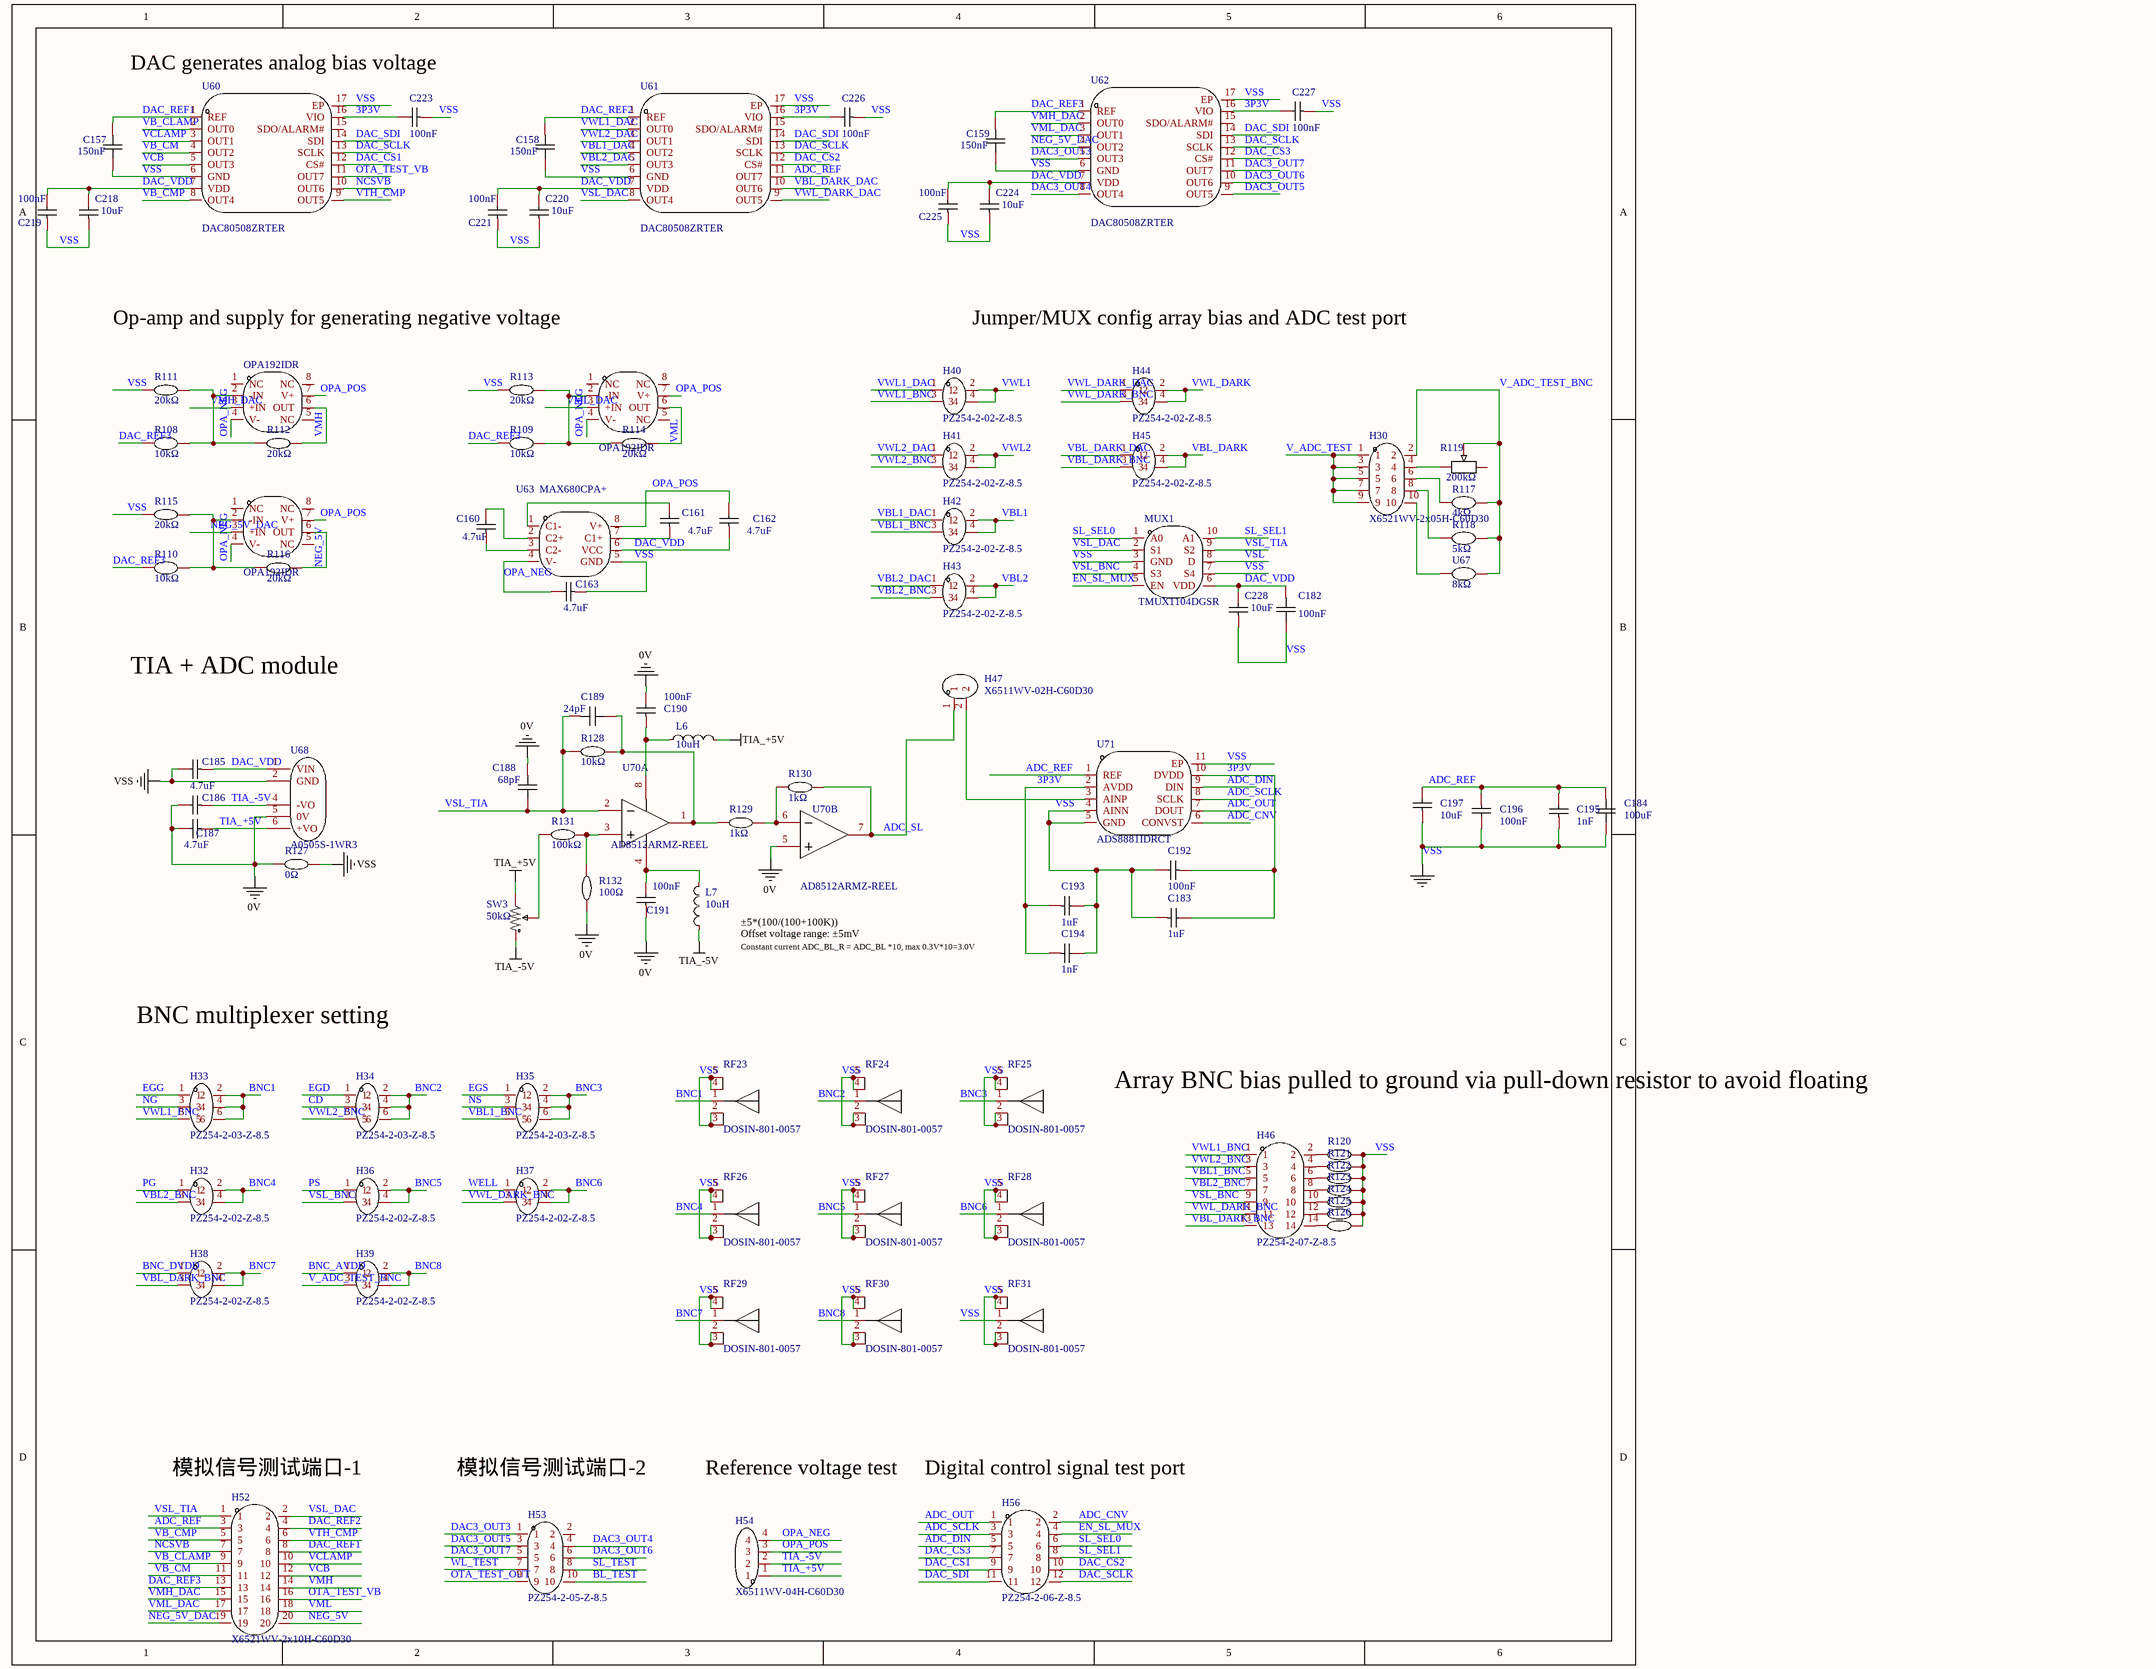
[diagram p0: MISC62793-4.schdoc]
# Altium project MISC62793-14.PrjPcb (part 3 of 4)
## Sheet MISC62793-4.schdoc (continued)
### Library data of the parts (continued)
R108-R110 = RT0603BRD0710KL: Manufacturer: YAGEO(国巨); Symbol: 1.25kΩ; Add into BOM: yes; Tolerance: ±0.1%; Power(Watts): 100mW; Overload Voltage (Max): 75V; Temperature Coefficient: ±25ppm/℃; Origin Footprint: R0805; Name: 10kΩ; Device: RT0603BRD0710KL; LCSC Part Name: 薄膜电阻 10kΩ ±0.1% 100mW; Supplier Part: C95204; Manufacturer Part: RT0603BRD0710KL; Supplier Footprint: 0603; JLCPCB Part Class: Extended Part; Datasheet: https://example.com/upload/public/pdf/source/20170217/1487301593756.pdf; Supplier: LCSC; Convert to PCB: yes; Type: Thin film resistor; Value: 10kΩ; Operating Temperature Range: -55℃~+155℃; Design Item ID: 1.25kΩ
R111-R116 = 0805W8F2002T5E: Manufacturer: UNI-ROYAL(厚声); Add into BOM: yes; Tolerance: ±1%; Power(Watts): 125mW; Overload Voltage (Max): 150V; Temperature Coefficient: ±100ppm/℃; Name: 20kΩ; Symbol: 0805W8F2002T5E; Device: 0805W8F2002T5E; Supplier: LCSC; Manufacturer Part: 0805W8F2002T5E; Supplier Part: C4328; Value: 20kΩ; JLCPCB Part Class: JLCPCB Part Class: Basic library; LCSC Part Name: 20kΩ ±1% 125mW 厚膜电阻; Supplier Footprint: 0805; Datasheet: https://example.com/upload/public/pdf/source/20200306/C422600_1E6D84923E4A46A82E41ADD87F860B5C.pdf; Convert to PCB: yes; Type: Thick film resistor; Operating Temperature Range: -55℃~+155℃
R117 = ARG05FTC4001N: Manufacturer: Viking(光颉); Add into BOM: yes; Tolerance: ±1%; Power(Watts): 125mW; Overload Voltage (Max): 150V; Temperature Coefficient: ±25ppm/℃; Name: 4kΩ; Symbol: ARG05FTC4001N; Device: ARG05FTC4001N; LCSC Part Name: 薄膜电阻 4kΩ ±1% 125mW; Supplier Part: C2828855; Manufacturer Part: ARG05FTC4001N; Supplier Footprint: 0805; JLCPCB Part Class: JLCPCB Part Class: Extended library; Datasheet: https://example.com/upload/public/pdf/source/20211009/C2828883_CAE7D170B8B230FC4A048BDC7B3A81FC.pdf; Supplier: LCSC; Convert to PCB: yes; Type: Thin film resistor; Value: 4kΩ; Operating Temperature Range: -55℃~+155℃
R118 = ARG05BTC5001N: Manufacturer: Viking(光颉); Add into BOM: yes; Tolerance: ±0.1%; Power(Watts): 125mW; Overload Voltage (Max): 150V; Temperature Coefficient: ±25ppm/℃; Name: 5kΩ; Symbol: ARG05BTC5001N; Device: ARG05BTC5001N; LCSC Part Name: 薄膜电阻 5kΩ ±0.1% 125mW; Supplier Part: C2828700; Manufacturer Part: ARG05BTC5001N; Supplier Footprint: 0805; JLCPCB Part Class: JLCPCB Part Class: Extended library; Datasheet: https://example.com/upload/public/pdf/source/20190816/C412422_E173BA386C6DD8245B6A88358EF9877A.pdf; Supplier: LCSC; Convert to PCB: yes; Type: Thin film resistor; Value: 5kΩ; Operating Temperature Range: -55℃~+155℃
R119 = ST-32EA 200K ohm (204): Manufacturer: NIDEC(尼得科); Add into BOM: yes; Tolerance: ±20%; Name: 200kΩ; Symbol: ST-32EA 200K ohm (204); Device: ST-32EA 200K ohm (204); LCSC Part Name: 200kΩ ±20%; Supplier Part: C132895; Manufacturer Part: ST-32EA 200K ohm (204); Supplier Footprint: SMD; JLCPCB Part Class: JLCPCB Part Class: Extended library; Datasheet: https://example.com/upload/public/pdf/source/20170930/C132923_1506736331375997276.pdf; Supplier: LCSC; Convert to PCB: yes; Value: 200kΩ
R120-R126 = 1206W4F1004T5E: Manufacturer: UNI-ROYAL(厚声); Add into BOM: yes; Tolerance: ±1%; Power(Watts): 250mW; Overload Voltage (Max): 200V; Temperature Coefficient: ±100ppm/℃; Name: 1MΩ; Symbol: 1206W4F1004T5E; Device: 1206W4F1004T5E; Supplier: LCSC; Manufacturer Part: 1206W4F1004T5E; Supplier Part: C17927; Value: 1MΩ; JLCPCB Part Class: JLCPCB Part Class: Basic library; LCSC Part Name: 1MΩ ±1% 250mW 厚膜电阻; Supplier Footprint: 1206; Datasheet: https://example.com/upload/public/pdf/source/20200306/C422600_1E6D84923E4A46A82E41ADD87F860B5C.pdf; Convert to PCB: yes; Type: Thick film resistor; Operating Temperature Range: -55℃~+155℃
R127 = 0603WAF0000T5E: Manufacturer: UNI-ROYAL(厚声); Add into BOM: yes; Tolerance: ±1%; Power(Watts): 100mW; Overload Voltage (Max): 75V; Name: 0Ω; Symbol: 0603WAF0000T5E; Device: 0603WAF0000T5E; Supplier: LCSC; Manufacturer Part: 0603WAF0000T5E; Supplier Part: C21189; Value: 0Ω; JLCPCB Part Class: JLCPCB Part Class: Basic library; LCSC Part Name: 0Ω ±1% 100mW 厚膜电阻; Supplier Footprint: 0603; Datasheet: https://example.com/upload/public/pdf/source/20200306/C422600_1E6D84923E4A46A82E41ADD87F860B5C.pdf; Convert to PCB: yes; Type: Thick film resistor; Operating Temperature Range: -55℃~+155℃
R128 = RT0603BRD0710KL: Manufacturer: YAGEO(国巨); Add into BOM: yes; Tolerance: ±0.1%; Power(Watts): 100mW; Overload Voltage (Max): 75V; Temperature Coefficient: ±25ppm/℃; Name: 10kΩ; Symbol: RT0603BRD0710KL; Device: RT0603BRD0710KL; LCSC Part Name: 薄膜电阻 10kΩ ±0.1% 100mW; Supplier Part: C95204; Manufacturer Part: RT0603BRD0710KL; Supplier Footprint: 0603; JLCPCB Part Class: Extended Part; Datasheet: https://example.com/upload/public/pdf/source/20170217/1487301593756.pdf; Supplier: LCSC; Convert to PCB: yes; Type: Thin film resistor; Value: 10kΩ; Operating Temperature Range: -55℃~+155℃
R129 R130 = RT0805BRD071KL: Manufacturer: YAGEO(国巨); Add into BOM: yes; Tolerance: ±0.1%; Power(Watts): 125mW; Overload Voltage (Max): 150V; Temperature Coefficient: ±25ppm/℃; Name: 1kΩ; Symbol: RT0805BRD071KL; Device: RT0805BRD071KL; LCSC Part Name: 薄膜电阻 1kΩ ±0.1% 125mW; Supplier Part: C110774; Manufacturer Part: RT0805BRD071KL; Supplier Footprint: 0805; JLCPCB Part Class: JLCPCB Part Class: Extended library; Datasheet: https://example.com/upload/public/pdf/source/20171026/C133380_15089840010201058857.pdf; Supplier: LCSC; Convert to PCB: yes; Type: Thin film resistor; Value: 1kΩ; Operating Temperature Range: -55℃~+155℃
R131 = RT0603BRD07100KL: Manufacturer: YAGEO(国巨); Add into BOM: yes; Tolerance: ±0.1%; Power(Watts): 100mW; Overload Voltage (Max): 75V; Temperature Coefficient: ±25ppm/℃; Name: 100kΩ; Symbol: RT0603BRD07100KL; Device: RT0603BRD07100KL; LCSC Part Name: 薄膜电阻 100kΩ ±0.1% 100mW; Supplier Part: C122538; Manufacturer Part: RT0603BRD07100KL; Supplier Footprint: 0603; JLCPCB Part Class: JLCPCB Part Class: Extended library; Datasheet: https://example.com/upload/public/pdf/source/20170721/C122538_1500619326323834092.pdf; Supplier: LCSC; Convert to PCB: yes; Type: Thin film resistor; Value: 100kΩ; Operating Temperature Range: -55℃~+155℃
R132 = RT0603BRD07100RL: Manufacturer: YAGEO(国巨); Add into BOM: yes; Tolerance: ±0.1%; Power(Watts): 100mW; Overload Voltage (Max): 75V; Temperature Coefficient: ±25ppm/℃; Name: 100Ω; Symbol: RT0603BRD07100RL; Device: RT0603BRD07100RL; LCSC Part Name: 薄膜电阻 100Ω ±0.1% 100mW; Supplier Part: C122970; Manufacturer Part: RT0603BRD07100RL; Supplier Footprint: 0603; JLCPCB Part Class: JLCPCB Part Class: Extended library; Datasheet: https://example.com/upload/public/pdf/source/20180716/C95646_694A11296E8D6C27B0592E54BC4097D1.pdf; Supplier: LCSC; Convert to PCB: yes; Type: Thin film resistor; Value: 100Ω; Operating Temperature Range: -55℃~+155℃
RF23-RF31 = DOSIN-801-0057: Manufacturer: dosinconn(德索五金); Add into BOM: yes; Connector Type: Board mount; Number of Ports: 1; Frequency-Max: 3GHz; RF Series: BNC; Impedance: 75Ω; Style: Straight pin; Name: DOSIN-801-0057; Symbol: DOSIN-801-0057; Device: DOSIN-801-0057; Supplier: LCSC; Supplier Part: C709675; Manufacturer Part: DOSIN-801-0057; JLCPCB Part Class: JLCPCB Part Class: Extended library; LCSC Part Name: BNC 正脚; Supplier Footprint: 插件; Datasheet: https://example.com/upload/public/pdf/source/20200723/C709675_AF24476B62C99F1B816FD550BCD101A8.pdf; Convert to PCB: yes; Interface Type: -; Interface Diameter: -; Interface Length/Height: -; Operating Temperature Range: -40℃~+110℃
SW3 = ST-5ETW503: Manufacturer: NIDEC(尼得科); Add into BOM: yes; Tolerance: ±10%; Power(Watts): 250mW; Temperature Coefficient: ±100ppm/℃; Turns: 14; Name: 50kΩ; Symbol: ST-5ETW503; Device: ST-5ETW503; LCSC Part Name: 50kΩ ±10%; Supplier Part: C2922110; Manufacturer Part: ST-5ETW503; Supplier Footprint: SMD; JLCPCB Part Class: JLCPCB Part Class: Extended library; Datasheet: https://example.com/upload/public/pdf/source/20220330/184EF06EE7E9D6CD77FC30947DCE7074.pdf; Supplier: LCSC; Convert to PCB: yes; Value: 50kΩ; Rated Voltage: -
U60-U62 = DAC80508ZRTER: Manufacturer: TI(德州仪器); Add into BOM: yes; Interface: SPI; Output Type: Voltage buffer; Supply Voltage: 1.7V~5.5V; Resolution: 16-bit; Integral nonlinearity: ±0.5LSB; ±0.5LSB; Settling Time: 5us; Name: DAC80508ZRTER; Symbol: DAC80508ZRTER; Device: DAC80508ZRTER; Supplier: LCSC; Supplier Part: C2679499; Manufacturer Part: DAC80508ZRTER; LCSC Part Name: DAC80508ZRTER; Supplier Footprint: WQFN-16-EP(3x3); Convert to PCB: yes; Operating Temperature: -40℃~+125℃
U63 = MAX680CPA+: Manufacturer: ADI(亚德诺)/MAXIM(美信); Add into BOM: yes; Output Type: Fixed; Input Voltage: 2V~6V; Output Voltage: -10V; 10V; Output Current (Max): 10mA; Switching Frequency: 8kHz; Synchronous Rectification: No; Number of Outputs: 2; Switch tube (built-in/external): Built-in; Name: MAX680CPA+; Symbol: MAX680CPA+; Device: MAX680CPA+; Supplier: LCSC; Manufacturer Part: MAX680CPA+; Supplier Part: C143569; JLCPCB Part Class: JLCPCB Part Class: Extended library; LCSC Part Name: MAX680CPA+; Supplier Footprint: DIP-8; Datasheet: https://example.com/upload/public/pdf/source/20171204/C143569_15123772720171162723.pdf; Convert to PCB: yes; Function: -; Operating Temperature: 0℃~+70℃@(TA); Topology: -
U64-U66 = OPA192IDR: Manufacturer: TI(德州仪器); Add into BOM: yes; Number of Circuits: Single channel; Gain Bandwidth Product(GBP): 10MHz; Current - Input Bias(Ib): 5pA; Slew Rate(SR): 20V/us; Output Current: 65mA; Name: OPA192IDR; Symbol: OPA192IDR; Device: OPA192IDR; Supplier: LCSC; Supplier Part: C2861286; Manufacturer Part: OPA192IDR; LCSC Part Name: OPA192IDR; Supplier Footprint: SOIC-8; Convert to PCB: yes; Output Type: -; Rail to Rail: -; Operating Temperature: -40℃~+125℃
U67 = 0805W8F8001T5E: Manufacturer: UNI-ROYAL(厚声); Add into BOM: yes; Tolerance: ±1%; Power(Watts): 125mW; Overload Voltage (Max): 150V; Temperature Coefficient: ±100ppm/℃; Name: 8kΩ; Symbol: 0805W8F8001T5E; Device: 0805W8F8001T5E; LCSC Part Name: 8kΩ ±1% 125mW 厚膜电阻; Supplier Part: C2767533; Manufacturer Part: 0805W8F8001T5E; Supplier Footprint: 0805; JLCPCB Part Class: JLCPCB Part Class: Extended library; Datasheet: https://example.com/upload/public/pdf/source/20200306/C422600_1E6D84923E4A46A82E41ADD87F860B5C.pdf; Supplier: LCSC; Convert to PCB: yes; Type: Thick film resistor; Value: 8kΩ; Operating Temperature Range: -55℃~+155℃
U68 = A0505S-1WR3_C131042: Manufacturer: MORNSUN(金升阳); Add into BOM: yes; Conversion Type: DC-DC; Input Voltage(DC): 4.5V~5.5V; Output Voltage: ±5V; Output Power: 1W; Output Current (Max): ±100mA; Output Channel: 2; Insulated Voltage: 1.5kV; Conversion Efficiency: 82%; Name: A0505S-1WR3; Symbol: A0505S-1WR3; Device: A0505S-1WR3_C131042; LCSC Part Name: A0505S-1WR3; Supplier Part: C131042; Manufacturer Part: A0505S-1WR3; Supplier Footprint: SIP,19.7x6mm; JLCPCB Part Class: JLCPCB Part Class: Extended library; Datasheet: https://example.com/upload/public/pdf/source/20170925/C131900_1506321486576990275.pdf; Supplier: LCSC; Convert to PCB: yes; Function: -
U70 = AD8512ARMZ-REEL: Manufacturer: ADI(亚德诺); Add into BOM: yes; Gain Bandwidth Product(GBP): 8MHz; Current - Input Bias(Ib): 25pA; Voltage - Input Offset(Vos): 100uV; Slew Rate(SR): 20V/us; Name: AD8512ARMZ-REEL; Symbol: AD8512ARMZ-REEL; Device: AD8512ARMZ-REEL; LCSC Part Name: AD8512ARMZ-REEL; Supplier Part: C36723; Manufacturer Part: AD8512ARMZ-REEL; Supplier Footprint: MSOP-8; JLCPCB Part Class: JLCPCB Part Class: Extended library; Datasheet: https://example.com/upload/public/pdf/source/20141125/1457707250819.pdf; Supplier: LCSC; Convert to PCB: yes; Operating Temperature: -40℃~+125℃
U71 = ADS8881IDRCT: Manufacturer: TI(德州仪器); Add into BOM: yes; Name: ADS8881IDRCT; Symbol: ADS8881IDRCT; Device: ADS8881IDRCT; LCSC Part Name: ADS8881IDRCT; Supplier Part: C2670688; Manufacturer Part: ADS8881IDRCT; Supplier Footprint: VSON-10-EP(3x3); JLCPCB Part Class: JLCPCB Part Class: Extended library; Supplier: LCSC; Convert to PCB: yes

## Sheet MISC62793-6.schdoc
size 185 x 185 mm; SheetNumber: 3; SheetTotal: 4
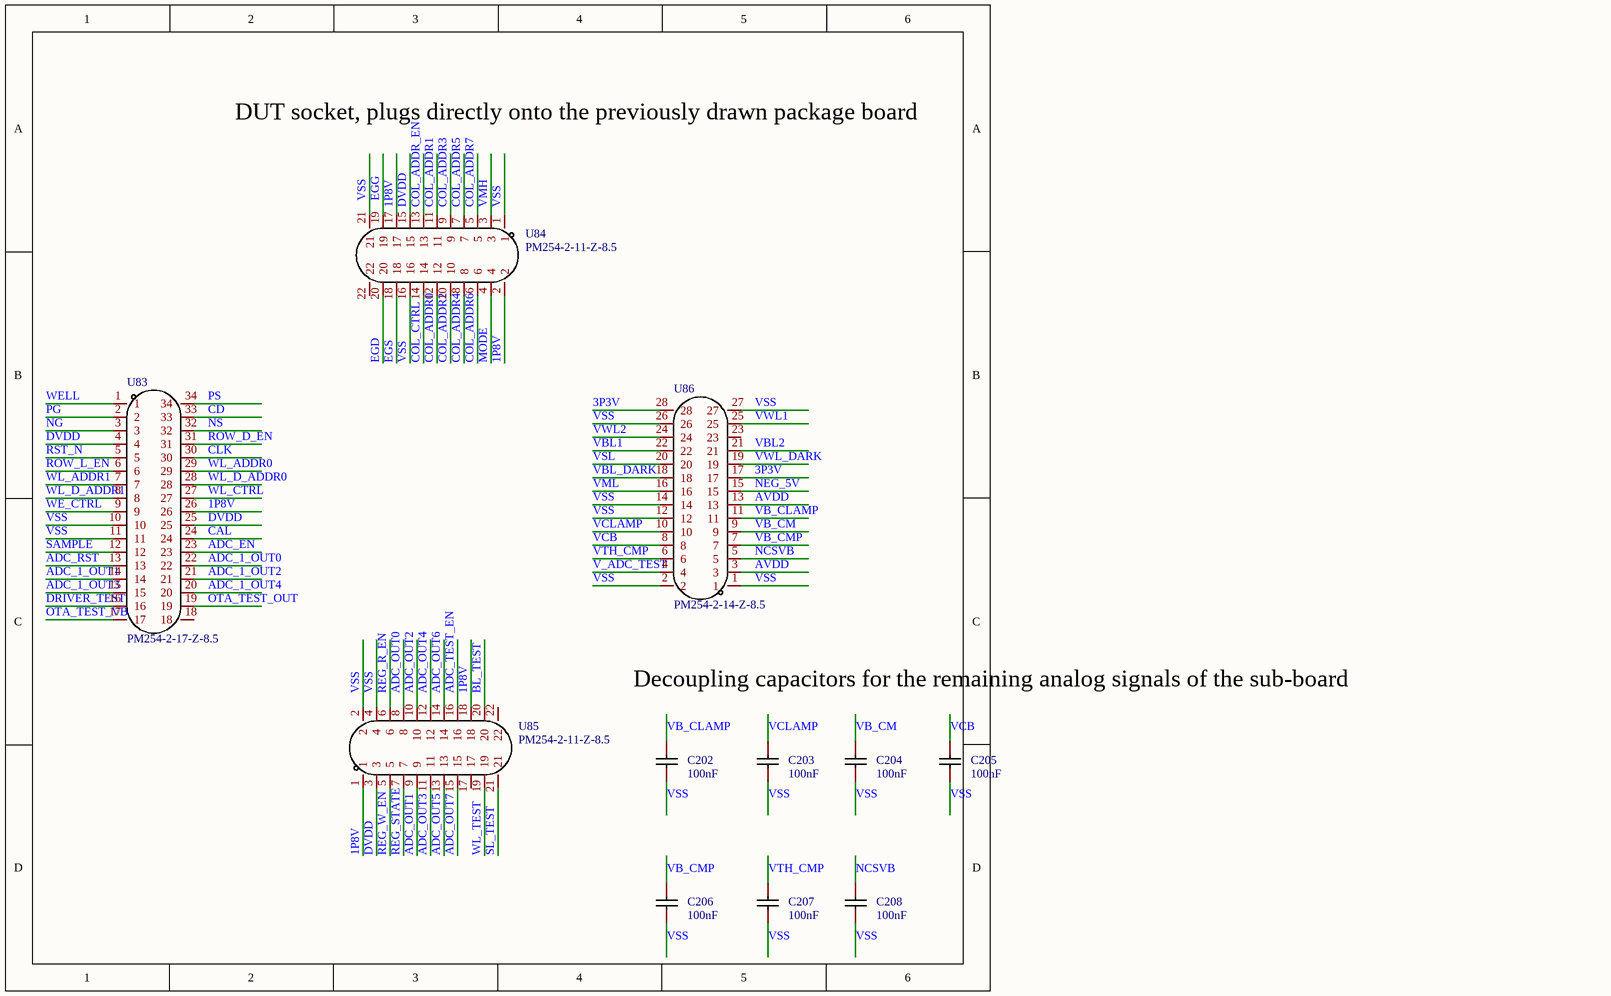
[diagram p1: MISC62793-6.schdoc]

### Parts
C202  100nF  [C0402]
C203  100nF  [C0402]
C204  100nF  [C0402]
C205  100nF  [C0402]
C206  100nF  [C0402]
C207  100nF  [C0402]
C208  100nF  [C0402]
U83  PM254-2-17-Z-8.5  [HDR-TH_34P-P2.54-V-F-R2-C17-S2.54-1]
U84  PM254-2-11-Z-8.5  [HDR-TH_22P-P2.54-V-F-R2-C11-S2.54]
U85  PM254-2-11-Z-8.5  [HDR-TH_22P-P2.54-V-F-R2-C11-S2.54]
U86  PM254-2-14-Z-8.5  [HDR-TH_28P-P2.54-V-F-R2-C14-S2.54-1]

### Nets
VSS: C202.2 C203.2 C204.2 C205.2 C206.2 C207.2 C208.2 U83.10 U83.11 U84.1 U84.16 U84.21 U85.2 U85.4 U86.1 U86.2 U86.12 U86.14 U86.26 U86.27
1P8V: U83.26 U84.2 U84.17 U85.1 U85.18
3P3V: U86.17 U86.28
ADC_1_OUT0: U83.22
ADC_1_OUT1: U83.14
ADC_1_OUT2: U83.21
ADC_1_OUT3: U83.15
ADC_1_OUT4: U83.20
ADC_EN: U83.23
ADC_OUT0: U85.8
ADC_OUT1: U85.9
ADC_OUT2: U85.10
ADC_OUT3: U85.11
ADC_OUT4: U85.12
ADC_OUT5: U85.13
ADC_OUT6: U85.14
ADC_OUT7: U85.15
ADC_RST: U83.13
ADC_TEST_EN: U85.16
AVDD: U86.3 U86.13
BL_TEST: U85.20
CAL: U83.24
CD: U83.33
CLK: U83.30
COL_ADDR0: U84.12
COL_ADDR1: U84.11
COL_ADDR2: U84.10
COL_ADDR3: U84.9
COL_ADDR4: U84.8
COL_ADDR5: U84.7
COL_ADDR6: U84.6
COL_ADDR7: U84.5
COL_ADDR_EN: U84.13
COL_CTRL: U84.14
DRIVER_TEST: U83.16
DVDD: U83.4 U83.25 U84.15 U85.3
EGD: U84.20
EGG: U84.19
EGS: U84.18
MODE: U84.4
NCSVB: C208.1 U86.5
NEG_5V: U86.15
NG: U83.3
NS: U83.32
OTA_TEST_OUT: U83.19
OTA_TEST_VB: U83.17
PG: U83.2
PS: U83.34
REG_R_EN: U85.6
REG_STATE: U85.7
REG_W_EN: U85.5
ROW_D_EN: U83.31
ROW_L_EN: U83.6
RST_N: U83.5
SAMPLE: U83.12
SL_TEST: U85.21
V_ADC_TEST: U86.4
VB_CLAMP: C202.1 U86.11
VB_CM: C204.1 U86.9
VB_CMP: C206.1 U86.7
VBL1: U86.22
VBL2: U86.21
VBL_DARK: U86.18
VCB: C205.1 U86.8
VCLAMP: C203.1 U86.10
VMH: U84.3
VML: U86.16
VSL: U86.20
VTH_CMP: C207.1 U86.6
VWL1: U86.25
VWL2: U86.24
VWL_DARK: U86.19
WE_CTRL: U83.9
WELL: U83.1
WL_ADDR0: U83.29
WL_ADDR1: U83.7
WL_CTRL: U83.27
WL_D_ADDR0: U83.28
WL_D_ADDR1: U83.8
WL_TEST: U85.19

Not connected (* = marked no-connect by the designer): U83 18; U84 22; U85 17 22; U86 23

### Notes on the sheet
- DUT socket, plugs directly onto the previously drawn package board
- Decoupling capacitors for the remaining analog signals of the sub-board

### Library data of the parts
C202-C208 = CL05B104KO5NNNC: as C190-C192 on sheet MISC62793-4; Name: 100nF; Symbol: CL05B104KO5NNNC; Device: CL05B104KO5NNNC; Supplier: LCSC; Manufacturer Part: CL05B104KO5NNNC; Value: 100nF; Supplier Part: C1525; JLCPCB Part Class: JLCPCB Part Class: Basic library; LCSC Part Name: 100nF ±10% 16V; Supplier Footprint: 0402; Datasheet: https://example.com/upload/public/pdf/source/20160218/1457707763339.pdf; Convert to PCB: yes
U83 = PM254-2-17-Z-8.5: Manufacturer: HCTL(华灿天禄); Add into BOM: yes; Holes Structure: 2x17P; Pitch: 2.54mm; Circular Hole / Square Hole: Square hole; Number of Holes: 34P; Current Rating (Max): 3A; Holes Direction: Top; Soldering Temperature(Max): 260℃@5S; Name: PM254-2-17-Z-8.5; Symbol: PM254-2-17-Z-8.5; Device: PM254-2-17-Z-8.5; LCSC Part Name: 2x17P 间距:2.54mm 直插; Supplier Part: C2897418; Manufacturer Part: PM254-2-17-Z-8.5; Supplier Footprint: 插件,P=2.54mm; JLCPCB Part Class: JLCPCB Part Class: Extended library; Datasheet: https://example.com/upload/public/pdf/source/20230609/3D36CA2C1BFC9FD1C3F709AD9DFEB9C2.pdf; Supplier: LCSC; Convert to PCB: yes; Row Spacing: 2.54mm; Mounting Type: Through hole; Number of Rows: Dual row; Voltage Rating (Max): -; Insulation Height: 8.5mm; Contact Material: Copper alloy; Operating Temperature Range: -40℃~+105℃
U84 U85 = PM254-2-11-Z-8.5: Manufacturer: HCTL(华灿天禄); Add into BOM: yes; Holes Structure: 2x11P; Pitch: 2.54mm; Circular Hole / Square Hole: Square hole; Number of Holes: 22P; Current Rating (Max): 3A; Holes Direction: Top; Soldering Temperature(Max): 260℃@5S; Name: PM254-2-11-Z-8.5; Symbol: PM254-2-11-Z-8.5; Device: PM254-2-11-Z-8.5; LCSC Part Name: 2x11P 间距:2.54mm 直插; Supplier Part: C2897412; Manufacturer Part: PM254-2-11-Z-8.5; Supplier Footprint: 插件,P=2.54mm; JLCPCB Part Class: JLCPCB Part Class: Extended library; Datasheet: https://example.com/upload/public/pdf/source/20230609/3D36CA2C1BFC9FD1C3F709AD9DFEB9C2.pdf; Supplier: LCSC; Convert to PCB: yes; Row Spacing: 2.54mm; Mounting Type: Through hole; Number of Rows: Dual row; Voltage Rating (Max): -; Insulation Height: 8.5mm; Contact Material: Copper alloy; Operating Temperature Range: -40℃~+105℃
U86 = PM254-2-14-Z-8.5: Manufacturer: HCTL(华灿天禄); Add into BOM: yes; Holes Structure: 2x14P; Pitch: 2.54mm; Circular Hole / Square Hole: Square hole; Number of Holes: 28P; Current Rating (Max): 3A; Holes Direction: Top; Soldering Temperature(Max): 260℃@5S; Name: PM254-2-14-Z-8.5; Symbol: PM254-2-14-Z-8.5; Device: PM254-2-14-Z-8.5; LCSC Part Name: 2x14P 间距:2.54mm 直插; Supplier Part: C2897415; Manufacturer Part: PM254-2-14-Z-8.5; Supplier Footprint: 插件,P=2.54mm; JLCPCB Part Class: JLCPCB Part Class: Extended library; Datasheet: https://example.com/upload/public/pdf/source/20230609/3D36CA2C1BFC9FD1C3F709AD9DFEB9C2.pdf; Supplier: LCSC; Convert to PCB: yes; Row Spacing: 2.54mm; Mounting Type: Through hole; Number of Rows: Dual row; Voltage Rating (Max): -; Insulation Height: 8.5mm; Contact Material: Copper alloy; Operating Temperature Range: -40℃~+105℃

## Sheet MISC62793-8.schdoc
size 223 x 195 mm; SheetNumber: 4; SheetTotal: 4
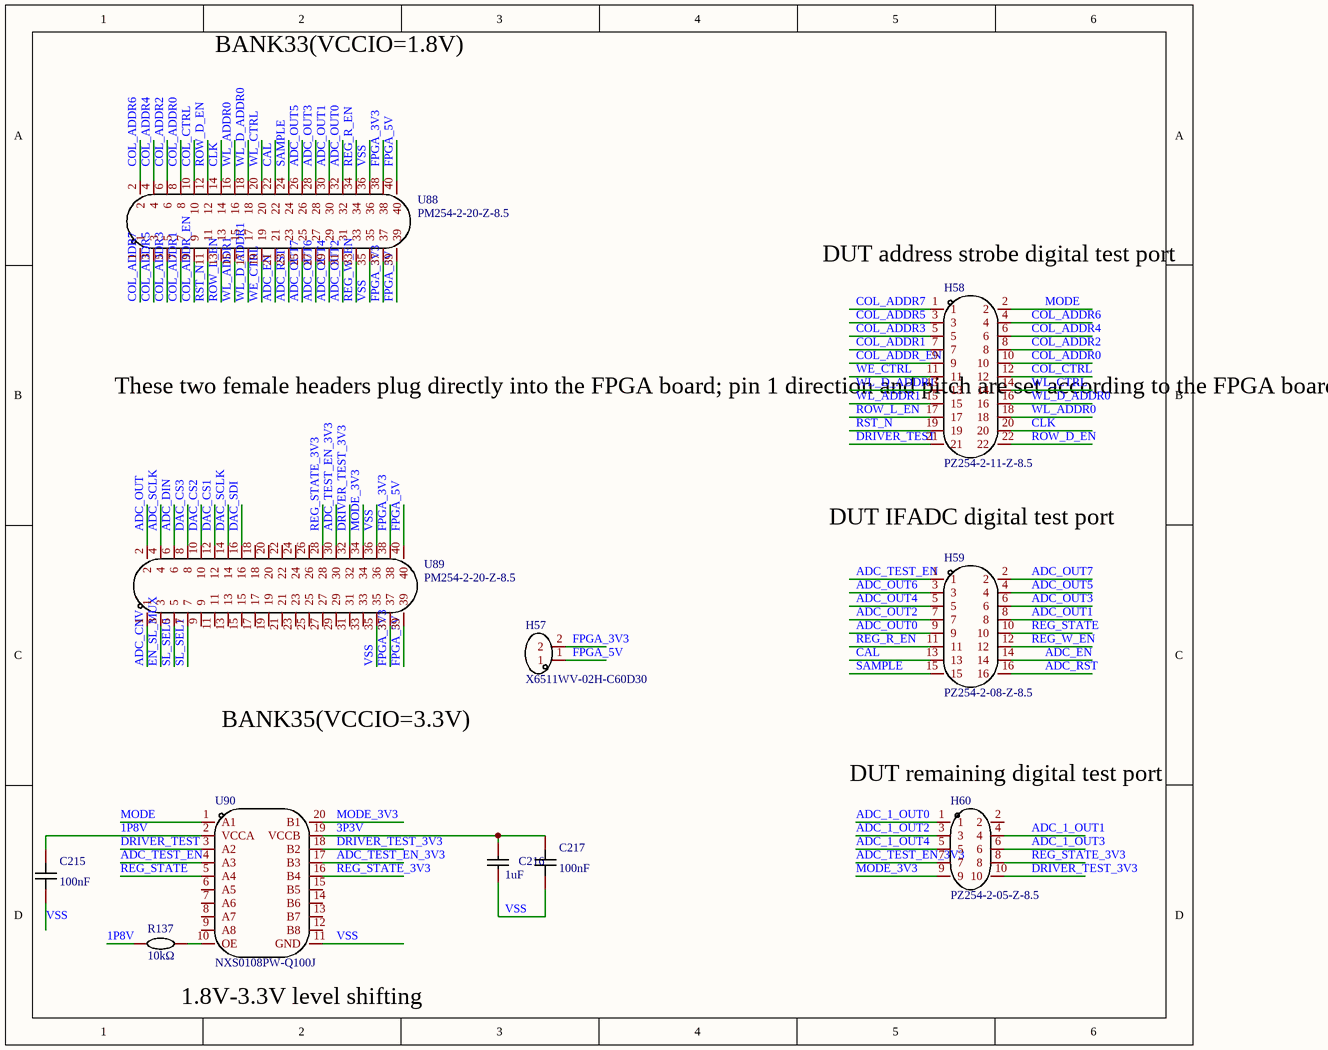
[diagram p2: MISC62793-8.schdoc]

### Parts
C215  100nF  [C0402]
C216  1uF  [C0603]
C217  100nF  [C0402]
H57  X6511WV-02H-C60D30  [HDR-TH_2P-P2.54-V-M]
H58  PZ254-2-11-Z-8.5  [HDR-TH_22P-P2.54-V-M-R2-C11-S2.54]
H59  PZ254-2-08-Z-8.5  [HDR-TH_16P-P2.54-V-M-R2-C8-S2.54]
H60  PZ254-2-05-Z-8.5  [HDR-TH_10P-P2.54-V-M-R2-C5-S2.54]
R137  10kΩ  [R0603]
U88  PM254-2-20-Z-8.5  [HDR-TH_40P-P2.54-V-F-R2-C20-S2.54]
U89  PM254-2-20-Z-8.5  [HDR-TH_40P-P2.54-V-F-R2-C20-S2.54]
U90  NXS0108PW-Q100J  [TSSOP-20_L6.5-W4.4-P0.65-LS6.4-BL]

### Nets
VSS: C215.1 C216.1 C217.1 U88.35 U88.36 U89.35 U89.36 U90.11(GND)
1P8V: C215.2 R137.1 U90.2(VCCA)
3P3V: C216.2 C217.2 U90.19(VCCB)
ADC_1_OUT0: H60.1
ADC_1_OUT1: H60.4
ADC_1_OUT2: H60.3
ADC_1_OUT3: H60.6
ADC_1_OUT4: H60.5
ADC_CNV: U89.1
ADC_DIN: U89.6
ADC_EN: H59.14 U88.21
ADC_OUT: U89.2
ADC_OUT0: H59.9 U88.32
ADC_OUT1: H59.8 U88.30
ADC_OUT2: H59.7 U88.31
ADC_OUT3: H59.6 U88.28
ADC_OUT4: H59.5 U88.29
ADC_OUT5: H59.4 U88.26
ADC_OUT6: H59.3 U88.27
ADC_OUT7: H59.2 U88.25
ADC_RST: H59.16 U88.23
ADC_SCLK: U89.4
ADC_TEST_EN: H59.1 U90.4(A3)
ADC_TEST_EN_3V3: H60.7 U89.30 U90.17(B3)
CAL: H59.13 U88.22
CLK: H58.20 U88.14
COL_ADDR0: H58.10 U88.8
COL_ADDR1: H58.7 U88.7
COL_ADDR2: H58.8 U88.6
COL_ADDR3: H58.5 U88.5
COL_ADDR4: H58.6 U88.4
COL_ADDR5: H58.3 U88.3
COL_ADDR6: H58.4 U88.2
COL_ADDR7: H58.1 U88.1
COL_ADDR_EN: H58.9 U88.9
COL_CTRL: H58.12 U88.10
DAC_CS1: U89.12
DAC_CS2: U89.10
DAC_CS3: U89.8
DAC_SCLK: U89.14
DAC_SDI: U89.16
DRIVER_TEST: H58.21 U90.3(A2)
DRIVER_TEST_3V3: H60.10 U89.32 U90.18(B2)
EN_SL_MUX: U89.3
FPGA_3V3: H57.2 U88.37 U88.38 U89.37 U89.38
FPGA_5V: H57.1 U88.39 U88.40 U89.39 U89.40
MODE: H58.2 U90.1(A1)
MODE_3V3: H60.9 U89.34 U90.20(B1)
REG_R_EN: H59.11 U88.34
REG_STATE: H59.10 U90.5(A4)
REG_STATE_3V3: H60.8 U89.28 U90.16(B4)
REG_W_EN: H59.12 U88.33
ROW_D_EN: H58.22 U88.12
ROW_L_EN: H58.17 U88.13
RST_N: H58.19 U88.11
SAMPLE: H59.15 U88.24
SL_SEL0: U89.5
SL_SEL1: U89.7
WE_CTRL: H58.11 U88.19
WL_ADDR0: H58.18 U88.16
WL_ADDR1: H58.15 U88.15
WL_CTRL: H58.14 U88.20
WL_D_ADDR0: H58.16 U88.18
WL_D_ADDR1: H58.13 U88.17
NetR137_2: R137.2 U90.10(OE)

Not connected (* = marked no-connect by the designer): H60 2; U89 9 11 13 15 17 18 19 20 21 22 23 24 25 26 27 29 31 33; U90 6(A5) 7(A6) 8(A7) 9(A8) 12(B8) 13(B7) 14(B6) 15(B5)

### Notes on the sheet
- BANK33(VCCIO=1.8V)
- (near H58) DUT address strobe digital test port
- These two female headers plug directly into the FPGA board; pin 1 direction and pitch are set according to the FPGA board
- DUT IFADC digital test port
- BANK35(VCCIO=3.3V)
- (near H60) DUT remaining digital test port
- 1.8V-3.3V level shifting

### Library data of the parts
C215 C217 = CC0402KRX7R7BB104: as C182 on sheet MISC62793-4; Name: 100nF; Symbol: CC0402KRX7R7BB104; Device: CC0402KRX7R7BB104; Supplier: LCSC; Manufacturer Part: CC0402KRX7R7BB104; Value: 100nF; Supplier Part: C60474; JLCPCB Part Class: JLCPCB Part Class: Extended library; LCSC Part Name: 100nF ±10% 16V; Supplier Footprint: 0402; Datasheet: https://example.com/upload/public/pdf/source/20211223/9278FD768280B81DDBEF48FA36411A03.pdf; Convert to PCB: yes
C216 = CL05A105KO5NNNC: Manufacturer: SAMSUNG(三星); Add into BOM: yes; Tolerance: ±10%; Voltage Rated: 16V; Temperature Coefficient: X5R; Name: 1uF; Symbol: CL05A105KO5NNNC; Device: CL05A105KO5NNNC; Supplier: LCSC; Manufacturer Part: CL05A105KO5NNNC; Value: 1uF; Supplier Part: C29266; JLCPCB Part Class: JLCPCB Part Class: Extended library; LCSC Part Name: 1uF ±10% 16V; Supplier Footprint: 0402; Datasheet: https://example.com/upload/public/pdf/source/20160218/1457707763339.pdf; Convert to PCB: yes
H57 = X6511WV-02H-C60D30: as H47 on sheet MISC62793-4; Name: X6511WV-02H-C60D30; Device: X6511WV-02H-C60D30; LCSC Part Name: 1x2P 间距:2.54mm 方针; Supplier Part: C706874; Manufacturer Part: X6511WV-02H-C60D30; Supplier Footprint: 插件,P=2.54mm; JLCPCB Part Class: JLCPCB Part Class: Extended library; Supplier: LCSC; Convert to PCB: yes; Row Spacing: 2.54mm; Mounting Type: -; Number of Rows: Single row; Number of Pins: 2P; Length of Mating Pin: 6mm; Insulation Height: 2.5mm; Length of End Connection Pin: 3mm; Contact Material: Brass; Contact Plating: Gold; Operating Temperature Range: -40℃~+105℃; Color: Black
H58 = PZ254-2-11-Z-8.5: Manufacturer: HCTL(华灿天禄); Add into BOM: yes; Pin Structure: 2x11P; Pitch: 2.54mm; Circluar Pins/Square Pins: Square pin; Current Rating (Max): 3A; Soldering Temperature(Max): 260℃@10S; Name: PZ254-2-11-Z-8.5; Symbol: PZ254-2-11-Z-8.5; Device: PZ254-2-11-Z-8.5; LCSC Part Name: 2x11P 间距:2.54mm 方针 直插; Supplier Part: C2894972; Manufacturer Part: PZ254-2-11-Z-8.5; Supplier Footprint: 插件,P=2.54mm; JLCPCB Part Class: JLCPCB Part Class: Extended library; Datasheet: https://example.com/upload/public/pdf/source/20230609/5BA09C8BEB9B31376F8BF6032FF67CAC.pdf; Supplier: LCSC; Convert to PCB: yes; Row Spacing: 2.54mm; Mounting Type: Through hole; Number of Rows: Dual row; Number of Pins: 22P; Voltage Rating (Max): -; Length of Mating Pin: 6mm; Insulation Height: 2.5mm; Length of End Connection Pin: 3mm; Contact Material: Brass; Operating Temperature Range: -40℃~+105℃; Color: Black
H59 = PZ254-2-08-Z-8.5: Manufacturer: HCTL(华灿天禄); Add into BOM: yes; Pin Structure: 2x8P; Pitch: 2.54mm; Circluar Pins/Square Pins: Square pin; Current Rating (Max): 3A; Soldering Temperature(Max): 260℃@10S; Name: PZ254-2-08-Z-8.5; Symbol: PZ254-2-08-Z-8.5; Device: PZ254-2-08-Z-8.5; LCSC Part Name: 2x8P 间距:2.54mm 方针 直插; Supplier Part: C2894969; Manufacturer Part: PZ254-2-08-Z-8.5; Supplier Footprint: 插件,P=2.54mm; JLCPCB Part Class: JLCPCB Part Class: Extended library; Datasheet: https://example.com/upload/public/pdf/source/20230609/5BA09C8BEB9B31376F8BF6032FF67CAC.pdf; Supplier: LCSC; Convert to PCB: yes; Row Spacing: 2.54mm; Mounting Type: Through hole; Number of Rows: Dual row; Number of Pins: 16P; Voltage Rating (Max): -; Length of Mating Pin: 6mm; Insulation Height: 2.5mm; Length of End Connection Pin: 3mm; Contact Material: Brass; Operating Temperature Range: -40℃~+105℃; Color: Black
H60 = PZ254-2-05-Z-8.5_C2894966: as H53 on sheet MISC62793-4; Name: PZ254-2-05-Z-8.5; Symbol: PZ254-2-05-Z-8.5; Device: PZ254-2-05-Z-8.5_C2894966; LCSC Part Name: 2x5P 间距:2.54mm 方针 直插; Supplier Part: C2894966; Manufacturer Part: PZ254-2-05-Z-8.5; Supplier Footprint: 插件,P=2.54mm; JLCPCB Part Class: JLCPCB Part Class: Extended library; Datasheet: https://example.com/upload/public/pdf/source/20230609/5BA09C8BEB9B31376F8BF6032FF67CAC.pdf; Supplier: LCSC; Convert to PCB: yes; Row Spacing: 2.54mm; Mounting Type: Through hole; Number of Rows: Dual row; Number of Pins: 10P; Voltage Rating (Max): -; Length of Mating Pin: 6mm; Insulation Height: 2.5mm; Length of End Connection Pin: 3mm; Contact Material: Brass; Operating Temperature Range: -40℃~+105℃; Color: Black
R137 = RT0603BRD0710KL: as R128 on sheet MISC62793-4; Name: 10kΩ; Symbol: RT0603BRD0710KL; Device: RT0603BRD0710KL; LCSC Part Name: 薄膜电阻 10kΩ ±0.1% 100mW; Supplier Part: C95204; Manufacturer Part: RT0603BRD0710KL; Supplier Footprint: 0603; JLCPCB Part Class: Extended Part; Datasheet: https://example.com/upload/public/pdf/source/20170217/1487301593756.pdf; Supplier: LCSC; Convert to PCB: yes; Type: Thin film resistor; Value: 10kΩ; Operating Temperature Range: -55℃~+155℃
U88 U89 = PM254-2-20-Z-8.5: Manufacturer: HCTL(华灿天禄); Add into BOM: yes; Holes Structure: 2x20P; Pitch: 2.54mm; Circular Hole / Square Hole: Square hole; Number of Holes: 40P; Current Rating (Max): 3A; Holes Direction: Top; Soldering Temperature(Max): 260℃@5S; Name: PM254-2-20-Z-8.5; Symbol: PM254-2-20-Z-8.5; Device: PM254-2-20-Z-8.5; LCSC Part Name: 2x20P 间距:2.54mm 直插; Supplier Part: C2897421; Manufacturer Part: PM254-2-20-Z-8.5; Supplier Footprint: 插件,P=2.54mm; JLCPCB Part Class: JLCPCB Part Class: Extended library; Datasheet: https://example.com/upload/public/pdf/source/20230609/3D36CA2C1BFC9FD1C3F709AD9DFEB9C2.pdf; Supplier: LCSC; Convert to PCB: yes; Row Spacing: 2.54mm; Mounting Type: Through hole; Number of Rows: Dual row; Voltage Rating (Max): -; Insulation Height: 8.5mm; Contact Material: Copper alloy; Operating Temperature Range: -40℃~+105℃
U90 = NXS0108PW-Q100J: Manufacturer: Nexperia(安世); Add into BOM: yes; Channel Type: Bidirectional; Data Rate: 110Mbps; Supply Voltage (VCCA): 1.2V~3.6V; Supply Voltage (VCCB): 1.65V~5.5V; Number of Circuits: 1; Channels per Circuit: 8; Output Type: Open drain; Name: NXS0108PW-Q100J; Symbol: NXS0108PW-Q100J; Device: NXS0108PW-Q100J; LCSC Part Name: NXS0108PW-Q100J; Supplier Part: C5361349; Manufacturer Part: NXS0108PW-Q100J; Supplier Footprint: TSSOP-20; JLCPCB Part Class: JLCPCB Part Class: Extended library; Datasheet: https://example.com/upload/public/pdf/source/20230504/D9F9E88A0217CE40025FEB7B2A59D4BA.pdf; Supplier: LCSC; Convert to PCB: yes; Operating Temperature: -40℃~+125℃